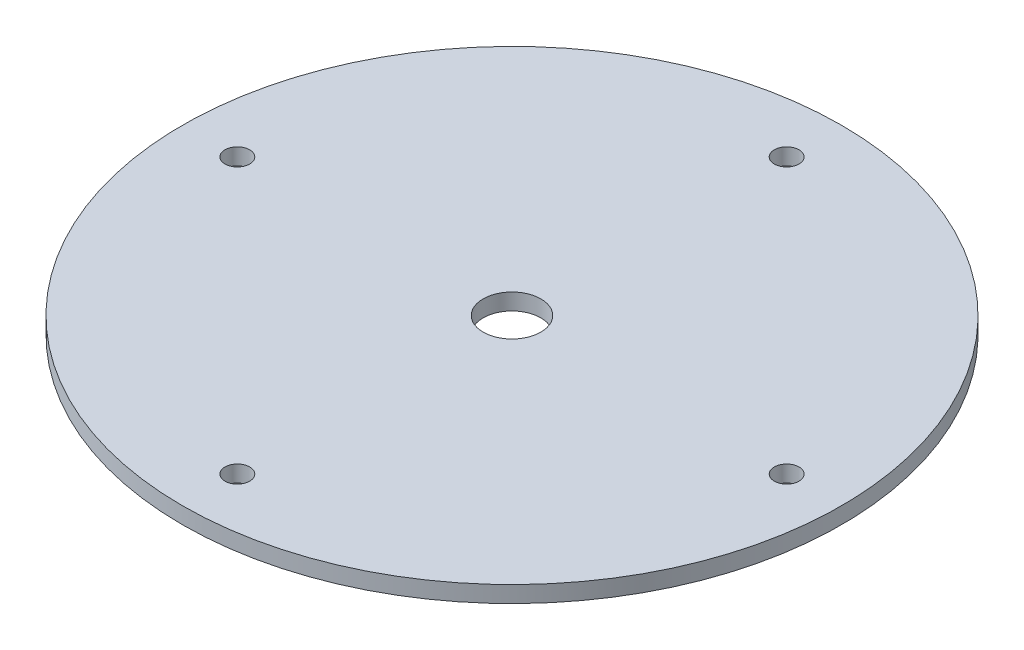
from build123d import *

# Parameters (mm, degrees)
SKETCH1_R           = 40
BOSS_EXTRUDE1_DEPTH = 2
SKETCH2_R           = 3.5
CUT_EXTRUDE3_DEPTH  = 52
SKETCH3_R           = 1.5
CUT_EXTRUDE4_DEPTH  = 45


with BuildPart() as part:
    # Sketch1 → Boss-Extrude1 (new body)
    with BuildSketch(Plane(origin=(0, 0, 0), x_dir=(1, 0, 0), z_dir=(0, 1, 0))):
        with Locations(Location((0, 0, 0), (0, 0, 270))):
            Circle(SKETCH1_R)
    extrude(amount=BOSS_EXTRUDE1_DEPTH)

    # Sketch2 → Cut-Extrude3 (cut)
    with BuildSketch(Plane.XZ):
        with Locations(Location((0, 0, 0), (0, 0, 270))):
            Circle(SKETCH2_R)
    extrude(amount=-CUT_EXTRUDE3_DEPTH, mode=Mode.SUBTRACT)

    # Sketch3 → Cut-Extrude4 (cut)
    with BuildSketch(Plane(origin=(0, 2, 0), x_dir=(1, 0, 0), z_dir=(0, 1, 0))):
        with Locations(Location((0, 33.338700108, 0), (0, 0, 270))):
            Circle(SKETCH3_R)
        with Locations(Location((33.338700108, 0, 0), (0, 0, 270))):
            Circle(SKETCH3_R)
        with Locations(Location((0, -33.338700108, 0), (0, 0, 270))):
            Circle(SKETCH3_R)
        with Locations(Location((-33.338700108, 0, 0), (0, 0, 270))):
            Circle(SKETCH3_R)
    extrude(amount=-CUT_EXTRUDE4_DEPTH, mode=Mode.SUBTRACT)


solid = part.part
